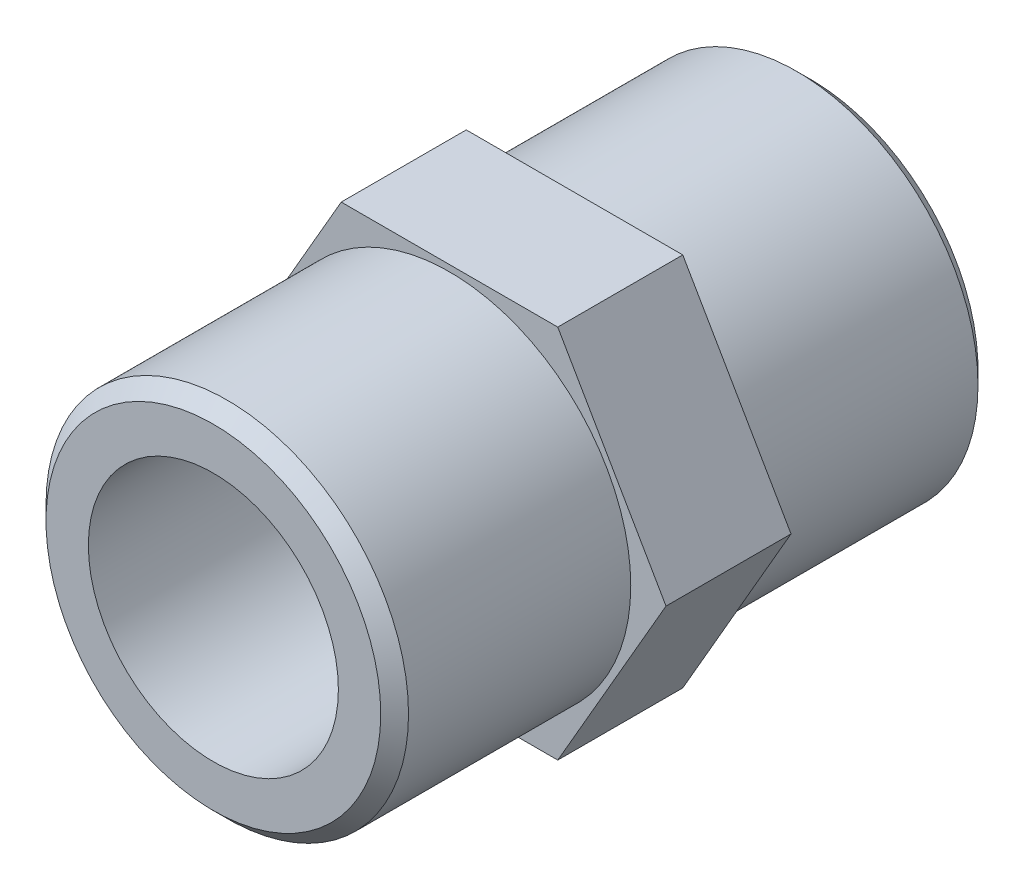
SolidWorks part; units mm, degrees
material "黄铜"
ref_plane "前视基准面" through (0, 0, 0) normal (0, 0, 1) x (1, 0, 0)
ref_plane "上视基准面" through (0, 0, 0) normal (0, 1, 0) x (1, 0, 0)
ref_plane "右视基准面" through (0, 0, 0) normal (1, 0, 0) x (0, 0, -1)
sketch "草图1" plane through (0, 0, 0) normal (0, 0, 1) x (1, 0, 0)
  line L0 (-1000, 0) -> (49000, 0) construction
  line L1 (15.5885, 0) -> (7.7942, 13.5)
  line L2 (7.7942, 13.5) -> (-7.7942, 13.5)
  line L3 (-7.7942, 13.5) -> (-15.5885, 0)
  line L4 (-15.5885, 0) -> (-7.7942, -13.5)
  line L5 (-7.7942, -13.5) -> (7.7942, -13.5)
  line L6 (7.7942, -13.5) -> (15.5885, 0)
  circle A0 centre (0, 0) radius 13.5 construction
  dimension "D1" = 27
extrude "凸台-拉伸1" add sketch "草图1" along normal mid plane 9
sketch "草图4" plane through (0, 0, -4.5) normal (0, 0, -1) x (-1, 0, 0)
  circle A0 centre (0, 0) radius 13.05
  dimension "D1" = 26.1
extrude "凸台-拉伸3" add sketch "草图4" along normal blind 17
cosmetic thread "装饰螺纹线2" parameters "D2"=18.631
mirror "镜向1" about plane through (0, 0, 0) normal (0, 0, 1) of "凸台-拉伸3"
sketch "草图5" plane through (0, 0, -21.5) normal (0, 0, -1) x (-1, 0, 0)
  circle A0 centre (0, 0) radius 9
  dimension "D1" = 18
extrude "切除-拉伸2" cut sketch "草图5" against normal up to next
chamfer "倒角1" distance 1 angle 45 2 edges at (-13.05, 0, -21.5) (-13.05, 0, 21.5)
